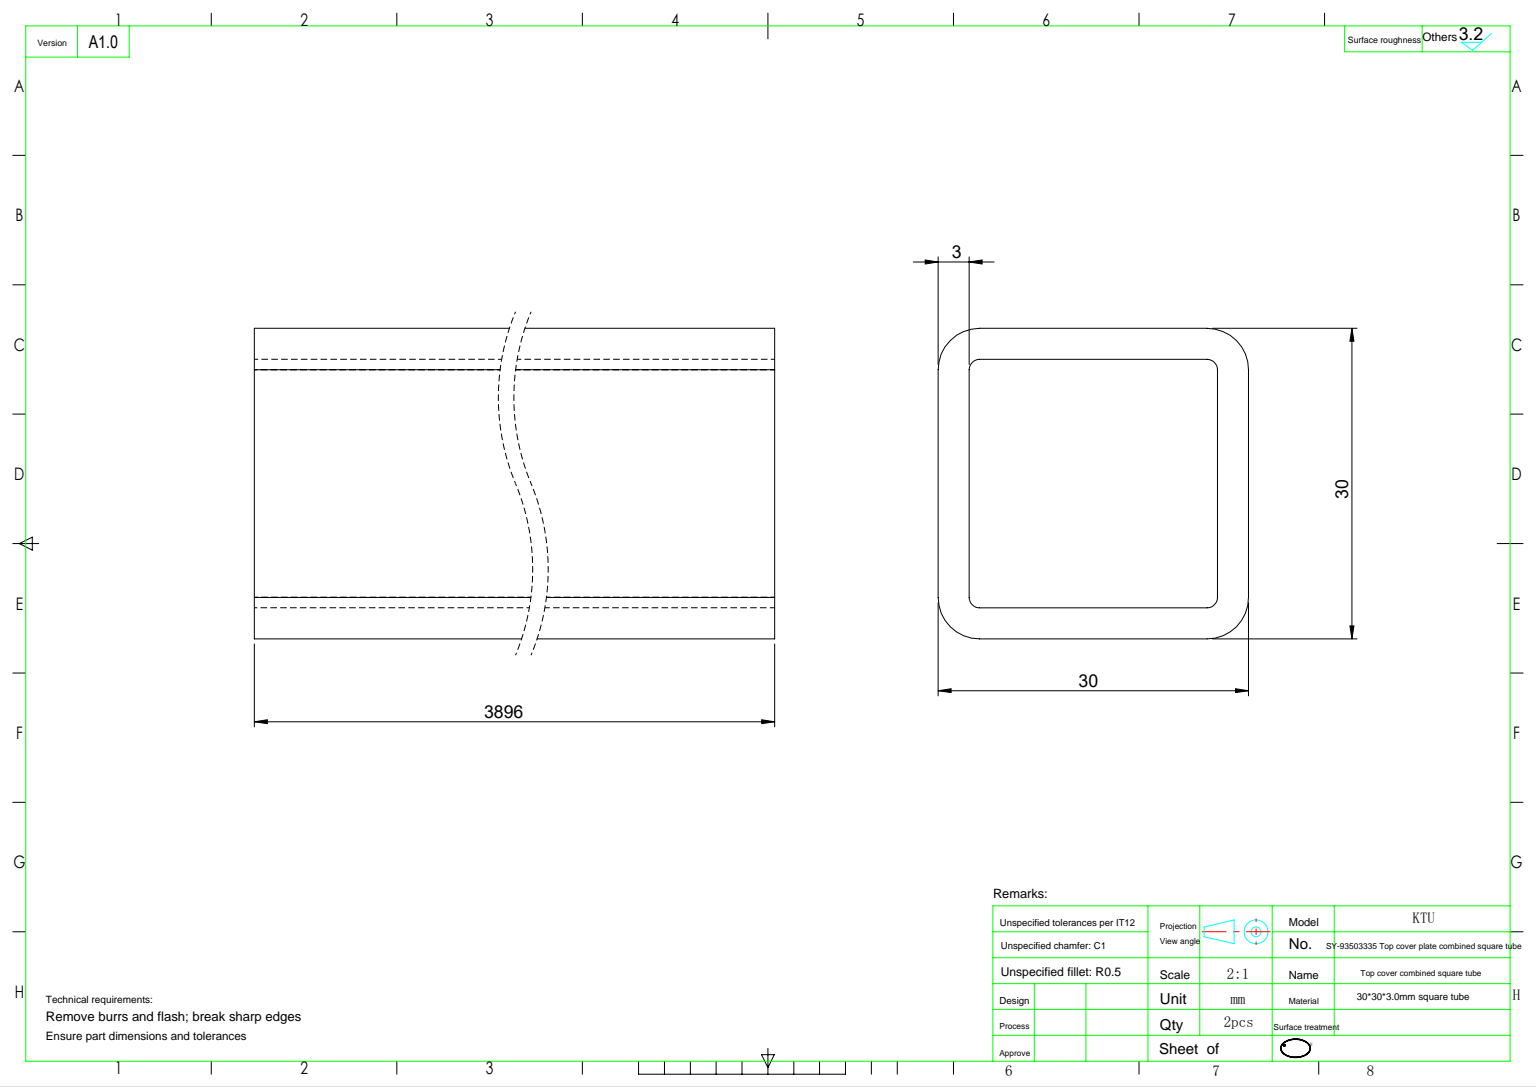
from build123d import *

# Parameters (mm, degrees)
EXTRUDE_1_DEPTH = 1948


with BuildPart() as part:
    # 草图2 → 拉伸-薄壁1 (new, symmetric)
    with BuildSketch(Plane.XY):
        with BuildLine():
            Line((-11, 15), (11, 15))
            ThreePointArc((11, 15), (13.828427125, 13.828427125), (15, 11))
            Line((15, 11), (15, -11))
            ThreePointArc((15, -11), (13.828427125, -13.828427125), (11, -15))
            Line((11, -15), (-11, -15))
            ThreePointArc((-11, -15), (-13.828427125, -13.828427125), (-15, -11))
            Line((-15, -11), (-15, 11))
            ThreePointArc((-15, 11), (-13.828427125, 13.828427125), (-11, 15))
        make_face()
        with BuildLine():
            Line((-11, 12), (11, 12))
            ThreePointArc((11, 12), (11.707106781, 11.707106781), (12, 11))
            Line((12, 11), (12, -11))
            ThreePointArc((12, -11), (11.707106781, -11.707106781), (11, -12))
            Line((11, -12), (-11, -12))
            ThreePointArc((-11, -12), (-11.707106781, -11.707106781), (-12, -11))
            Line((-12, -11), (-12, 11))
            ThreePointArc((-12, 11), (-11.707106781, 11.707106781), (-11, 12))
        make_face(mode=Mode.SUBTRACT)
    extrude(amount=EXTRUDE_1_DEPTH, both=True)


solid = part.part
